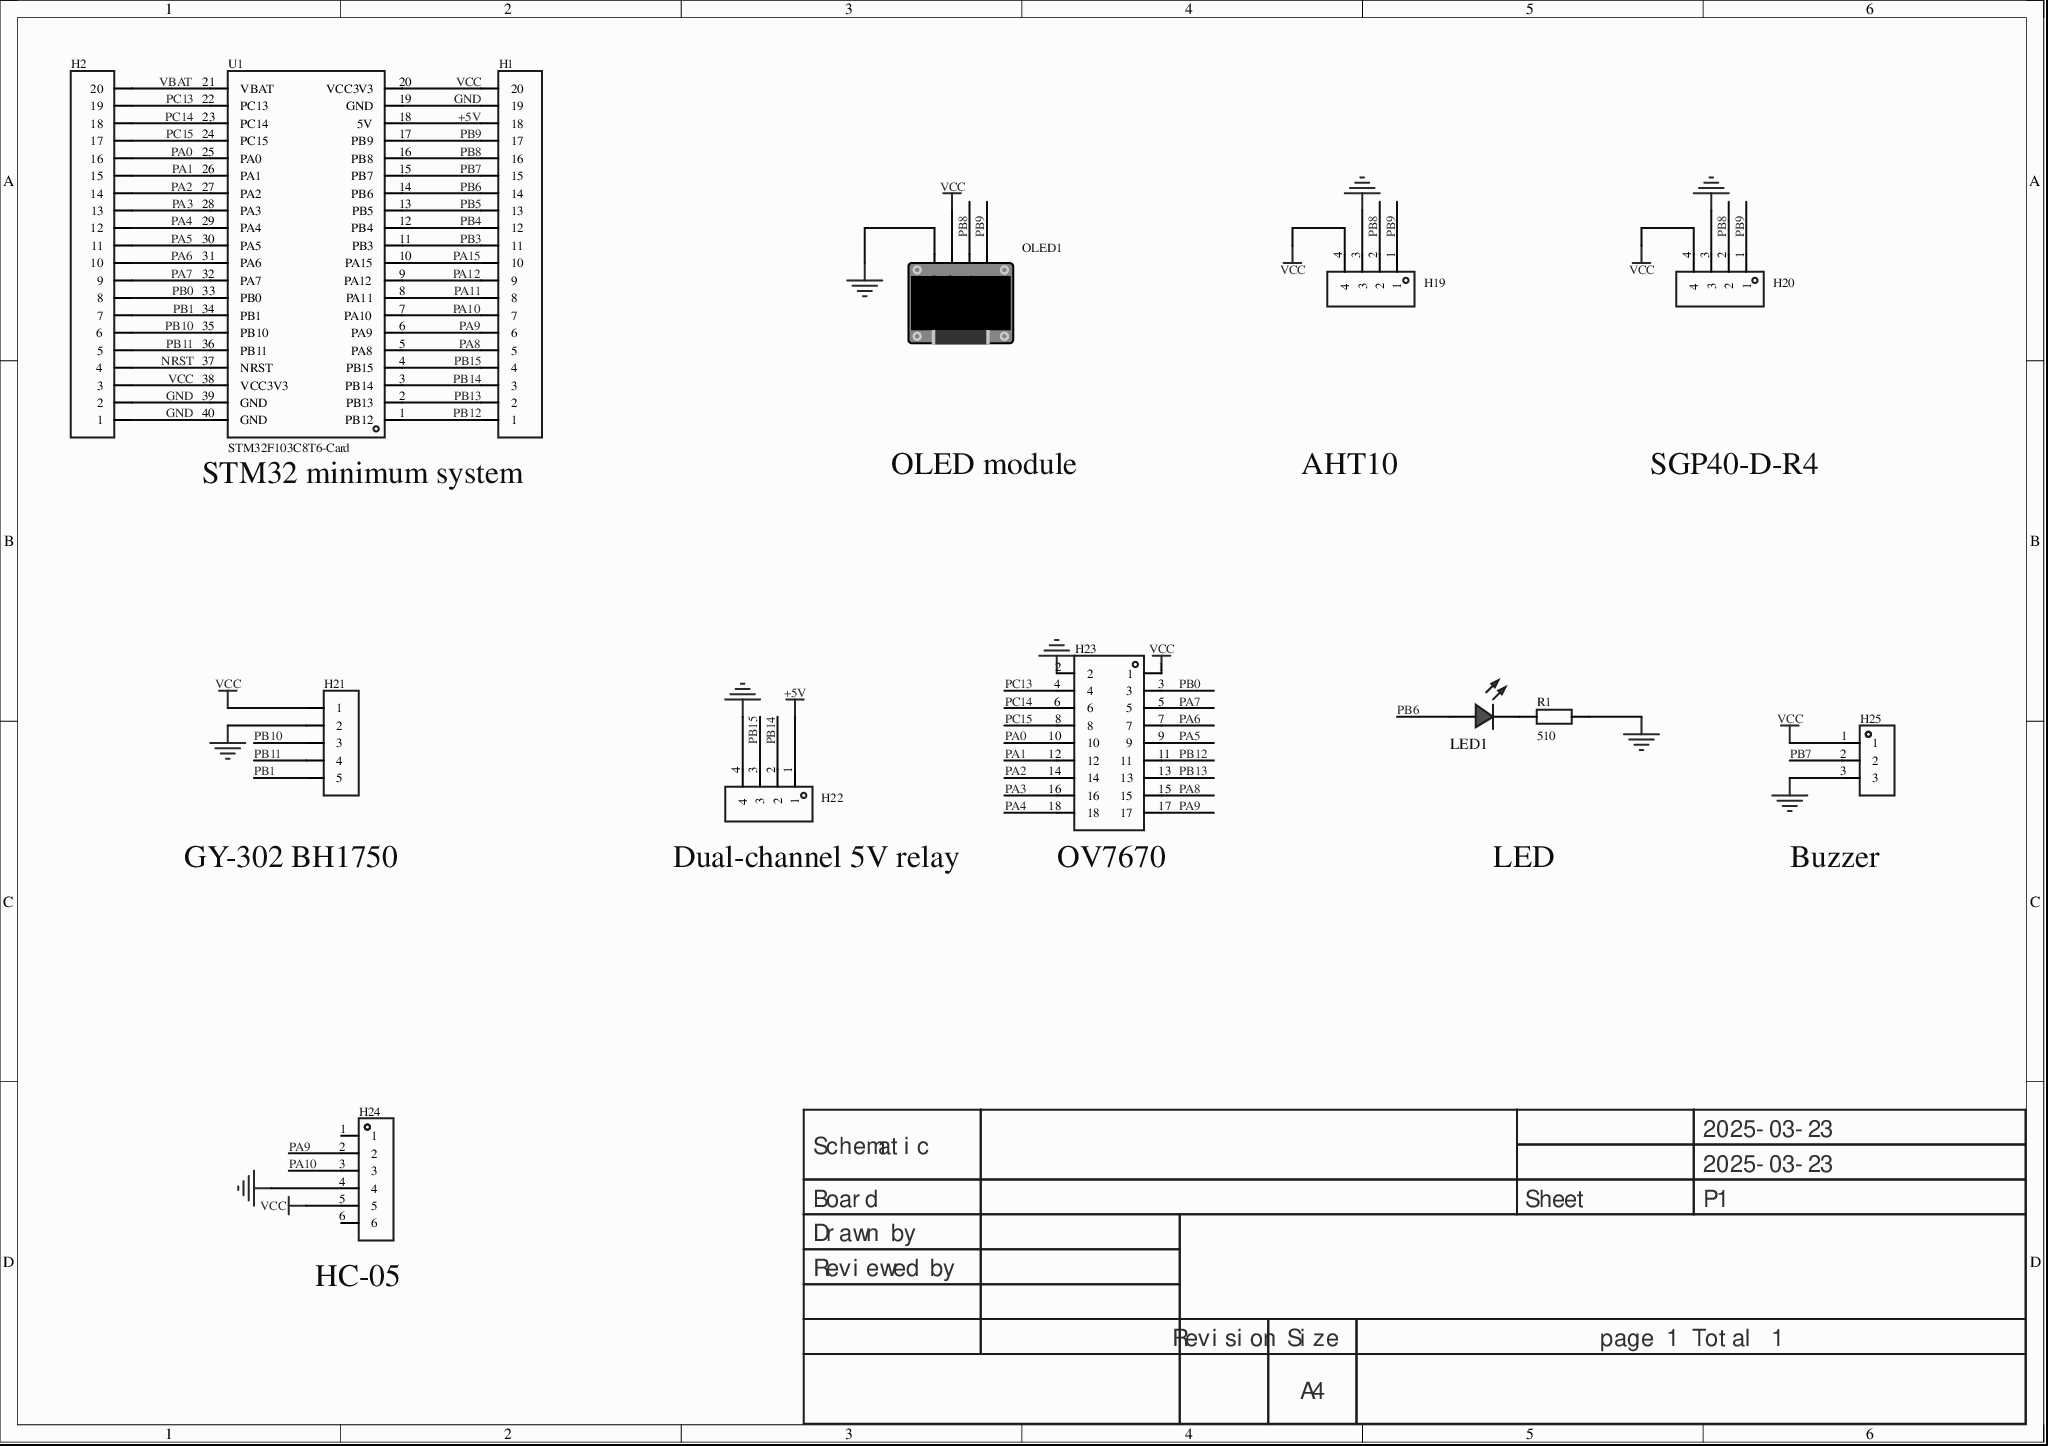
[diagram p0: MISC78996-3.schdoc]
# Altium project MISC78996-2.PrjPcb
1 sheet, 13 parts. Net scope: global (net labels, ports and power ports of the same name join across sheets).
Board file: MISC78996.pcbdoc

## Sheet MISC78996-3.schdoc
size 297 x 209 mm; Version: V1.0; @Project Name: MISC78996; @Page Count: 1; @Update Date: 2025-03-23; @Create Date: 2025-03-23; @Schematic Name: MISC78996; @Page No: 1; @Create Time: 15:37:32; @Update Time: 18:36:57; @Board Name: MISC78996

### Parts
H1  (no value)  [HDR-TH_20P-P2.54-V-F]
H2  (no value)  [HDR-TH_20P-P2.54-V-F]
H19  (no value)  [HDR-TH_4P-P2.54-V-F]
H20  (no value)  [HDR-TH_4P-P2.54-V-F]
H21  (no value)  [HDR-TH_5P-P2.54-V-F]
H22  (no value)  [HDR-TH_4P-P2.54-V-F]
H23  (no value)  [HDR-TH_18P-P2.54-V-M-R2-C9-S2.54]
H24  (no value)  [HDR-TH_6P-P2.54-V-F]
H25  (no value)  [HDR-TH_3P-P2.54-V-F]
LED1  (no value)  [LED_0603]
OLED1  (no value)  [0.96OLED_4P]
R1  510  [R0603]
U1  STM32F103C8T6-Card  [CONN-TH_L53.3-W22.9_STM32F103C8T6-CARD]

### Nets
+5V: H1.18 H22.1 U1.18(5V)
GND: H1.19 H2.1 H2.2 H19.3 H20.3 H21.2 H22.4 H23.2 H24.4 H25.3 OLED1.1(GND) R1.2 U1.19(GND) U1.39(GND) U1.40(GND)
VCC: H1.20 H2.3 H19.4 H20.4 H21.1 H23.1 H24.5 H25.1 OLED1.2(VCC) U1.20(VCC3V3) U1.38(VCC3V3)
NRST: H2.4 U1.37(NRST)
PA0: H2.16 H23.10 U1.25(PA0)
PA1: H2.15 H23.12 U1.26(PA1)
PA2: H2.14 H23.14 U1.27(PA2)
PA3: H2.13 H23.16 U1.28(PA3)
PA4: H2.12 H23.18 U1.29(PA4)
PA5: H2.11 H23.9 U1.30(PA5)
PA6: H2.10 H23.7 U1.31(PA6)
PA7: H2.9 H23.5 U1.32(PA7)
PA8: H1.5 H23.15 U1.5(PA8)
PA9: H1.6 H23.17 H24.2 U1.6(PA9)
PA10: H1.7 H24.3 U1.7(PA10)
PA11: H1.8 U1.8(PA11)
PA12: H1.9 U1.9(PA12)
PA15: H1.10 U1.10(PA15)
PB0: H2.8 H23.3 U1.33(PB0)
PB1: H2.7 H21.5 U1.34(PB1)
PB3: H1.11 U1.11(PB3)
PB4: H1.12 U1.12(PB4)
PB5: H1.13 U1.13(PB5)
PB6: H1.14 LED1.2(A) U1.14(PB6)
PB7: H1.15 H25.2 U1.15(PB7)
PB8: H1.16 H19.2 H20.2 OLED1.3(SCL) U1.16(PB8)
PB9: H1.17 H19.1 H20.1 OLED1.4(SDA) U1.17(PB9)
PB10: H2.6 H21.3 U1.35(PB10)
PB11: H2.5 H21.4 U1.36(PB11)
PB12: H1.1 H23.11 U1.1(PB12)
PB13: H1.2 H23.13 U1.2(PB13)
PB14: H1.3 H22.2 U1.3(PB14)
PB15: H1.4 H22.3 U1.4(PB15)
PC13: H2.19 H23.4 U1.22(PC13)
PC14: H2.18 H23.6 U1.23(PC14)
PC15: H2.17 H23.8 U1.24(PC15)
VBAT: H2.20 U1.21(VBAT)
NetLED1_1: LED1.1(C) R1.1

Not connected (* = marked no-connect by the designer): H24 1* 6*

### Notes on the sheet
- STM32 minimum system
- OLED module
- AHT10
- SGP40-D-R4
- (near H21) GY-302 BH1750
- Dual-channel 5V relay
- (near H23) OV7670
- LED
- (near H25) Buzzer
- (near H24) HC-05
- 2025-03-23
- Schematic
- Board
- Sheet
- P1
- Drawn by
- Reviewed by
- Revision
- Size
- A4
- page 1 Total 1

### Library data of the parts
H1 H2 = HDR-F_2.54_1x20P: ConvertToPcb: yes; ModelId: db7015f7ad9d48b8a3b1188db02e3429; ModelName: HDR-F-2.54_1x20; ModelTransform: 1999.996,100,0,0,0,0,0,0,-118.11; Device: HDR-F_2.54_1x20P; Symbol: HDR-F_2.54_1x20P; AddInBom: yes; SupplierPart: C50984; Supplier Footprint: 插件; FootprintName: HDR-TH_20P-P2.54-V-F
H19 H20 H22 = HDR-F_2.54_1x4P: ConvertToPcb: yes; SymbolName: 2.54-1*4P female; ModelId: d187812051054f85879fcaa51a310d8e; ModelTransform: 419.6842,98.464,0,0,0,0,0,0,-118.11; Device: HDR-F_2.54_1x4P; AddInBom: yes; SupplierPart: C2718488; Supplier Footprint: 插件; FootprintName: HDR-TH_4P-P2.54-V-F; ModelName: HDR-TH_4P-P2.54-V-F
H21 = HDR-F_2.54_1x5P: Symbol: Header-Female-2.54_1x5; ConvertToPcb: yes; ModelId: f49cb6116a3d45e5a64915bf3e00773f; ModelTransform: 519.684,98.464,0,0,0,0,0,0,-124.016; Device: HDR-F_2.54_1x5P; AddInBom: yes; SupplierPart: C50950; Supplier Footprint: 插件; FootprintName: HDR-TH_5P-P2.54-V-F; ModelName: HDR-TH_5P-P2.54-V-F
H23 = HDR-M_2.54_2x9: Symbol: HDR-M-2.54_2x9; ConvertToPcb: yes; ModelId: 7f5f7e3c551d46aa986089ba4aec6522; ModelName: HDR-TH_18P-P2.54-M-LI-2X9P; ModelTransform: 899.9982,200,0,0,0,0,0,0,-118.11; Device: HDR-M_2.54_2x9; AddInBom: yes; SupplierPart: C492426; Supplier Footprint: 插件,P=2.54mm; FootprintName: HDR-TH_18P-P2.54-V-M-R2-C9-S2.54
H24 = HDR-F_2.54_1x6P: Symbol: Header-Female-2.54_1x6; ConvertToPcb: yes; ModelId: 0f5bcf94dcda47d085f24cdca1696fe9; ModelTransform: 619.684,94.488,0,0,0,0,0,0,-125.984; Device: HDR-F_2.54_1x6P; AddInBom: yes; SupplierPart: C40877; Supplier Footprint: 插件; FootprintName: HDR-TH_6P-P2.54-V-F; ModelName: HDR-TH_6P-P2.54-V-F
H25 = HDR-F_2.54_1x3P: Symbol: PM254V-11-03-H85; ConvertToPcb: yes; ModelId: f3b3cc5aae9641bf9e56fc160cef875b; ModelName: HDR2.54-F-LI-1X3P; ModelTransform: 299.9994,100,0,0,0,0,0,0,-118.11; Device: HDR-F_2.54_1x3P; AddInBom: yes; SupplierPart: C541850; Supplier Footprint: 插件; FootprintName: HDR-TH_3P-P2.54-V-F
LED1 = LED_0603-R: Symbol: LED_R; Convert to PCB: yes; 3D Model: dd8257b0d61a4cd7b68939a056e08095; 3D Model Transform: 58.72,29.4,22.03,0,0,0,0,0,0; ModelName: LED-0603_R; Device: LED_0603-R; Add into BOM: yes; Supplier Footprint: 0603; FootprintName: LED_0603
OLED1 = 0.96OLED模块_4P: Device: 0.96OLED module_4P; ConvertToPcb: yes; ModelId: 79c000fdb68d45a296c2e9bedf4f9055; ModelTransform: 1393.69792,1318.895,0,0,0,0,0,-560.079,-137.795; AddInBom: yes; SymbolName: 0.96OLED module_4P; FootprintName: 0.96OLED_4P; Supplier Footprint: 插件; ModelName: 0.96OLED_4P
R1 = Res_0603: ConvertToPcb: yes; SymbolName: Resistor; ModelId: fc143cca1e79419f9cd78b61e9279f08; ModelTransform: 31.8897,63.7794,0,90,0,0,0,0,0; Value: 510; Device: Res_0603; AddInBom: yes; Supplier Footprint: 0603; FootprintName: R0603; ModelName: R0603
U1 = STM32F103C8T6-Card: AddInBom: yes; Symbol: STM32F103C8T6-CARD; Device: STM32F103C8T6-Card; LCSC Part Name: STM32F103C8T6-Card; SupplierPart: C9900077949; ManufacturerPart: STM32F103C8T6-Card; Supplier Footprint: 插件; Supplier: LCSC; ConvertToPcb: yes; FootprintName: CONN-TH_L53.3-W22.9_STM32F103C8T6-CARD